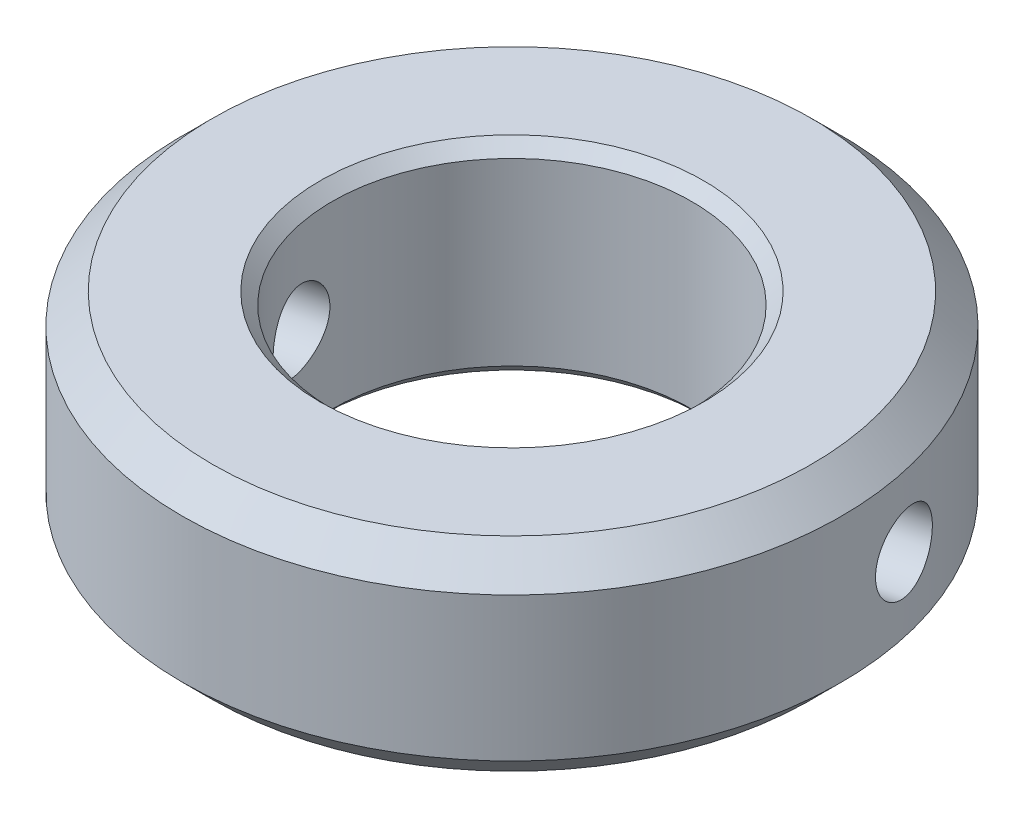
from build123d import *

# Parameters (mm, degrees)
SKETCH1_R                  = 55
SKETCH1_R_2                = 30
BOSS_EXTRUDE1_DEPTH        = 34
F_17_0_17_DIAMETER_HOLE1_D = 12.6
CHAMFER1_SIZE              = 5
CHAMFER2_SIZE              = 2


with BuildPart() as part:
    # Sketch1 → Boss-Extrude1 (new body)
    with BuildSketch(Plane(origin=(0, 0, 0), x_dir=(1, 0, 0), z_dir=(0, 1, 0))):
        with Locations(Location((0, 0, 0), (0, 0, 270))):
            Circle(SKETCH1_R)
        with Locations(Location((0, 0, 0), (0, 0, 270))):
            Circle(SKETCH1_R_2, mode=Mode.SUBTRACT)
    extrude(amount=BOSS_EXTRUDE1_DEPTH)

    # Ø17.0 (17) Diameter Hole1 (through all)
    with Locations(Plane(origin=(53.62356272, 17, -12.227572173), x_dir=(0.22231949406, 0, 0.97497386763), z_dir=(0.97497386763, 0, -0.22231949406))):
        with Locations((0, 0)):
            Hole(F_17_0_17_DIAMETER_HOLE1_D / 2)

    # Chamfer1
    chamfer1_edges = [part.edges().sort_by_distance(p)[0] for p in [
        (0, 0, -55),
        (0, 34, -55),
    ]]
    chamfer(chamfer1_edges, length=CHAMFER1_SIZE)

    # Chamfer2
    chamfer2_edges = [part.edges().sort_by_distance(p)[0] for p in [
        (0, 0, -30),
        (0, 34, -30),
    ]]
    chamfer(chamfer2_edges, length=CHAMFER2_SIZE)


solid = part.part
